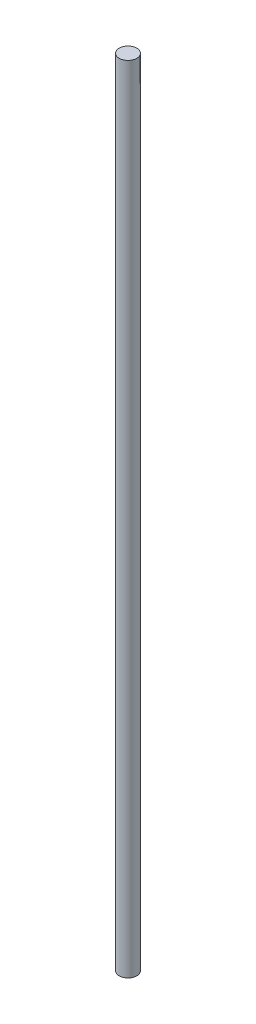
from build123d import *

# Parameters (mm, degrees)
SKETCH_1_R      = 2
EXTRUDE_1_DEPTH = 180


with BuildPart() as part:
    # 草图1 → 凸台-拉伸1 (new body)
    with BuildSketch(Plane(origin=(0, 0, 0), x_dir=(1, 0, 0), z_dir=(0, 1, 0))):
        with Locations(Location((0, 0, 0), (0, 0, 90))):
            Circle(SKETCH_1_R)
    extrude(amount=EXTRUDE_1_DEPTH)


solid = part.part
